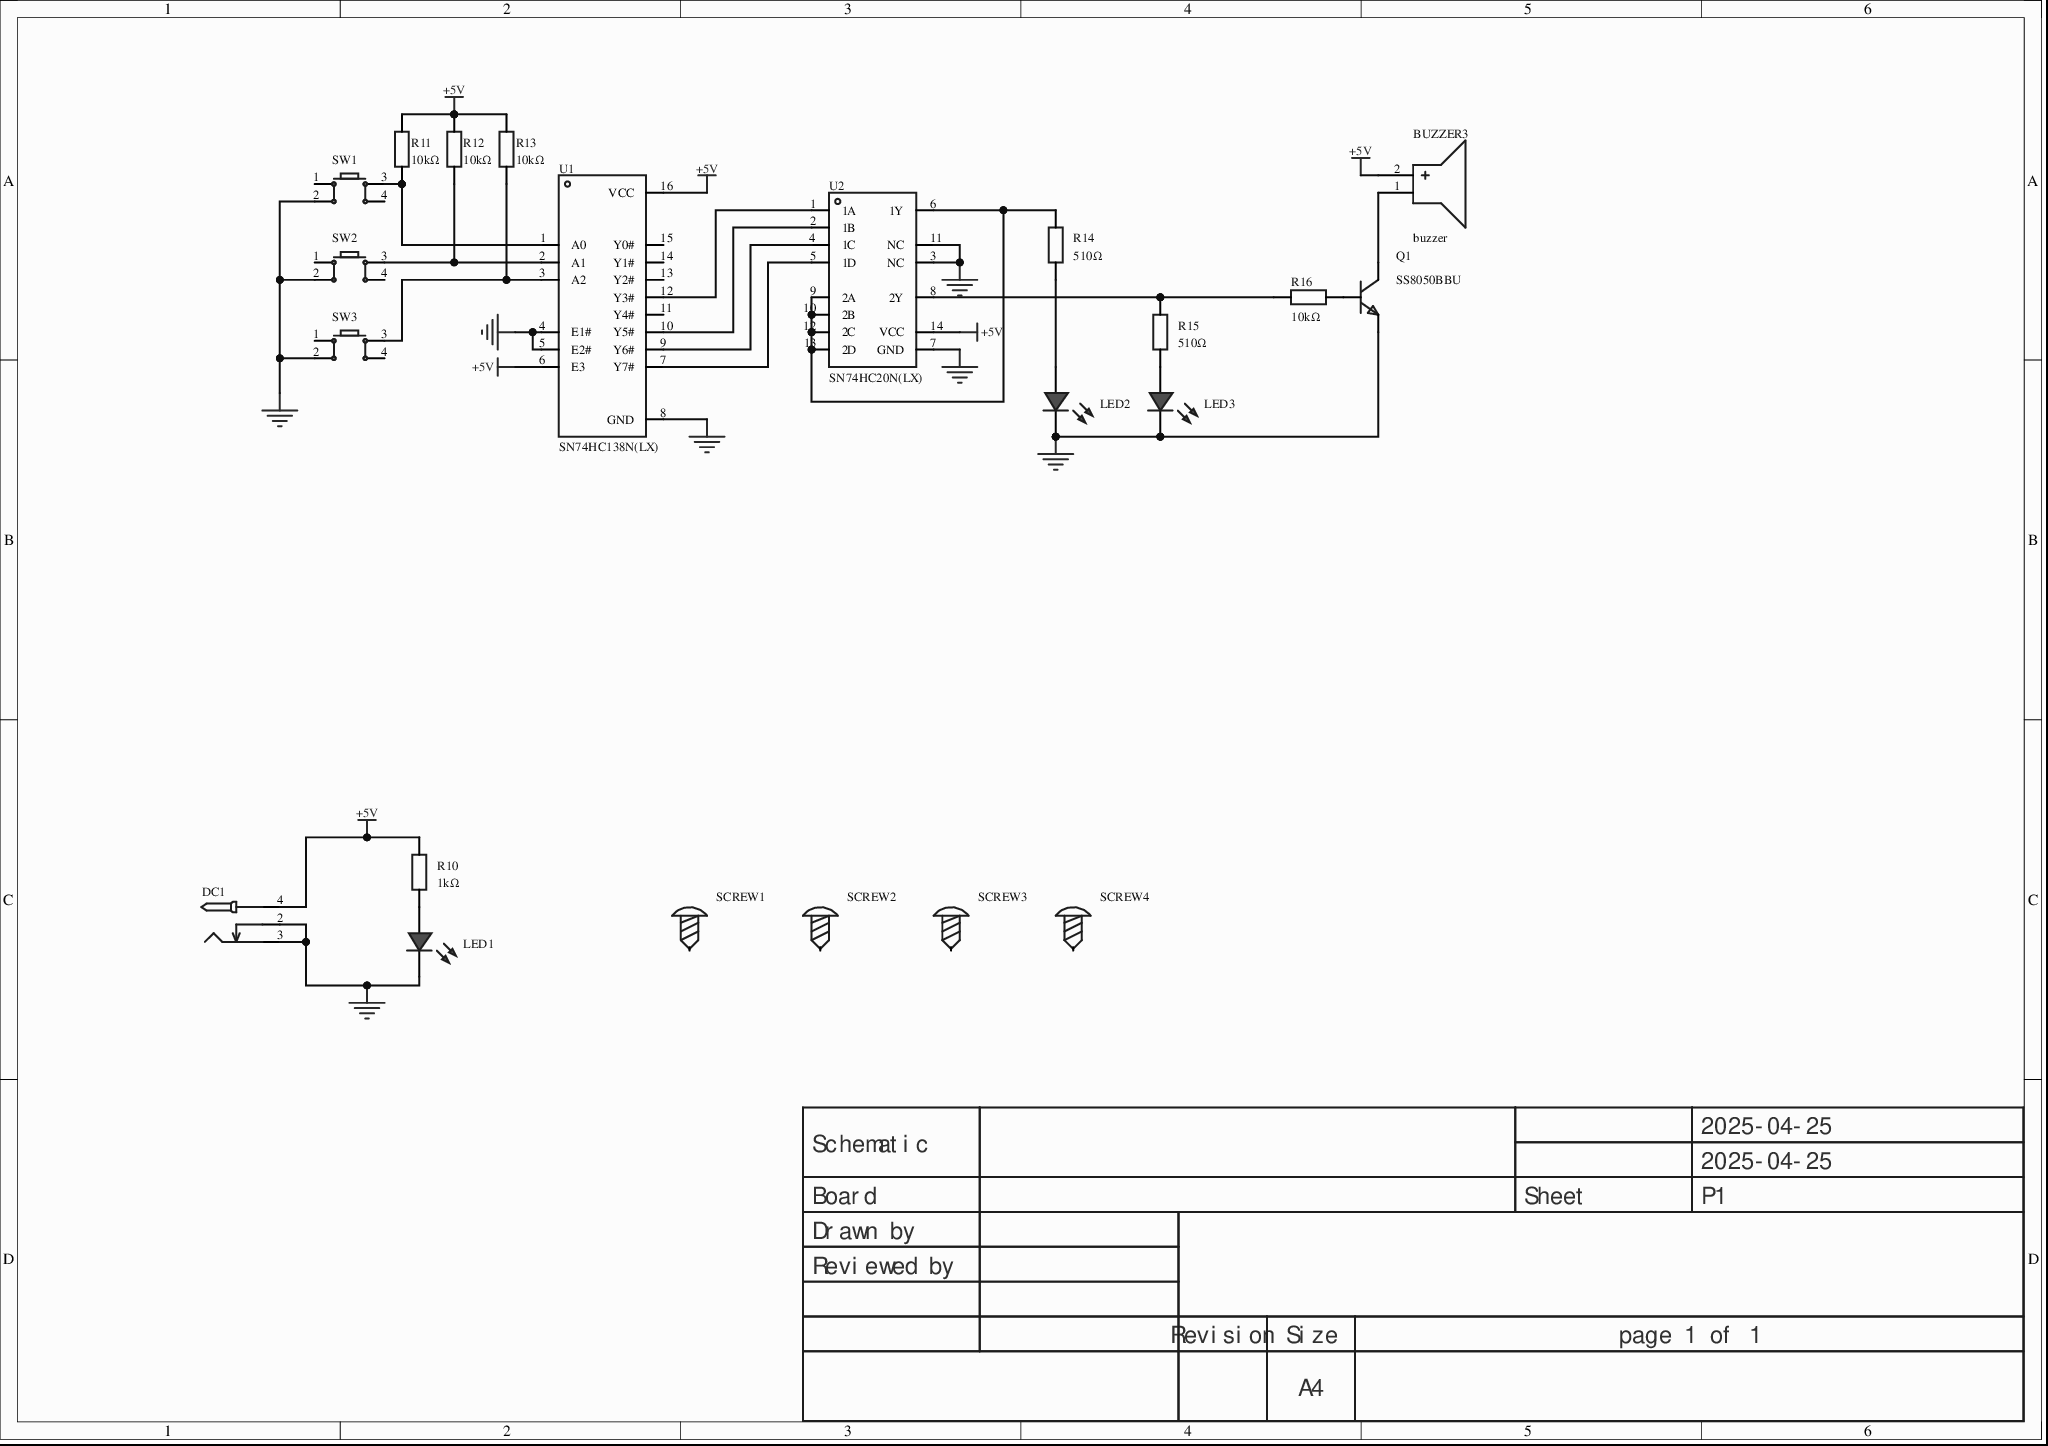
[diagram p0: MISC51615-3.schdoc]
# Altium project MISC51615-2.PrjPcb
1 sheet, 22 parts. Net scope: global (net labels, ports and power ports of the same name join across sheets).
Board file: MISC51615.pcbdoc

## Sheet MISC51615-3.schdoc
size 297 x 209 mm; Version: V1.0; @Project Name: MISC51615; @Page Count: 1; @Update Date: 2025-04-25; @Create Date: 2025-04-25; @Schematic Name: MISC51615; @Page No: 1; @Create Time: 10:35:49; @Update Time: 10:35:54; @Board Name: MISC51615

### Parts
BUZZER3  buzzer  [BUZ-TH_BD12.0-P6.00-D0.9-RD]
DC1  (no value)  [DC-2.0]
LED1  (no value)  [LED_TH-3mm]
LED2  (no value)  [LED_TH-3mm]
LED3  (no value)  [LED_TH-3mm]
Q1  SS8050BBU  [TO-92-3_L4.8-W3.7-P1.27-L-1]
R10  1kΩ  [Res_1/8W]
R11  10kΩ  [Res_1/8W]
R12  10kΩ  [Res_1/8W]
R13  10kΩ  [Res_1/8W]
R14  510Ω  [Res_1/8W]
R15  510Ω  [Res_1/8W]
R16  10kΩ  [Res_1/8W]
SCREW1  (no value)  [M3螺丝]
SCREW2  (no value)  [M3螺丝]
SCREW3  (no value)  [M3螺丝]
SCREW4  (no value)  [M3螺丝]
SW1  (no value)  [SW-TH_4P-L6.0-W6.0-P4.50-LS6.5]
SW2  (no value)  [SW-TH_4P-L6.0-W6.0-P4.50-LS6.5]
SW3  (no value)  [SW-TH_4P-L6.0-W6.0-P4.50-LS6.5]
U1  SN74HC138N(LX)  [PDIP-16_L19.3-W6.4-P2.54-LS7.94-BL]
U2  SN74HC20N(LX)  [PDIP-14_L19.3-W6.5-P2.54-LS7.6-BL]

### Nets
+5V: BUZZER3.2(+) DC1.4 R10.2 R11.2 R12.2 R13.2 U1.6(E3) U1.16(VCC) U2.14(VCC)
GND: DC1.2 DC1.3 LED1.2(A) LED2.2(A) LED3.2(A) Q1.1(E) SW1.2 SW2.2 SW3.2 U1.4(E1#) U1.5(E2#) U1.8(GND) U2.3(NC) U2.7(GND) U2.11(NC)
NetBUZZER3_1: BUZZER3.1(-) Q1.3(C)
NetLED1_1: LED1.1(C) R10.1
NetLED2_1: LED2.1(C) R14.1
NetLED3_1: LED3.1(C) R15.1
NetQ1_2: Q1.2(B) R16.2
NetR11_1: R11.1 SW1.3 U1.1(A0)
NetR12_1: R12.1 SW2.3 U1.2(A1)
NetR13_1: R13.1 SW3.3 U1.3(A2)
NetR14_2: R14.2 U2.6(1Y) U2.9(2A) U2.10(2B) U2.12(2C) U2.13(2D)
NetR15_2: R15.2 R16.1 U2.8(2Y)
NetU1_7: U1.7(Y7#) U2.5(1D)
NetU1_9: U1.9(Y6#) U2.4(1C)
NetU1_10: U1.10(Y5#) U2.2(1B)
NetU1_12: U1.12(Y3#) U2.1(1A)

Not connected (* = marked no-connect by the designer): SCREW1 1; SCREW2 1; SCREW3 1; SCREW4 1; SW1 1 4; SW2 1 4; SW3 1 4; U1 11(Y4#)* 13(Y2#)* 14(Y1#)* 15(Y0#)*

### Notes on the sheet
- 2025-04-25
- Schematic
- Board
- Sheet
- P1
- Drawn by
- Reviewed by
- Revision
- Size
- A4
- page 1 of 1

### Library data of the parts
BUZZER3 = buzzer: AddInBom: yes; ModelId: af17e4151ed84fc2a628230bf2376363; ModelTransform: 472.44,472.176,0,270,0,0,0,0,-196.85; Symbol: BUZZER; Device: buzzer; LCSC Part Name: buzzer; SupplierPart: C9900014030; ManufacturerPart: buzzer; Supplier Footprint: buzzer; JLCPCB Part Class: extended library; Supplier: LCSC; ConvertToPcb: yes; FootprintName: BUZ-TH_BD12.0-P6.00-D0.9-RD; ModelName: BUZ-TH_BD12.0-P6.00-D0.9-RD
DC1 = DC-005_2.0: ConvertToPcb: yes; SymbolName: DC power connector; ModelId: f5f20b8a2308479b936ba3c2698865bb0819f05c4eef4c71ace90d822a990e87; ModelName: DC-IN-TH_DC-5520-1; ModelTransform: 372.05,551.18,582.68,90,0,0,137.8,0,-149.61; Device: DC-005_2.0; AddInBom: yes; Supplier Footprint: 插件; FootprintName: DC-2.0
LED1-LED3 = LED_TH-R_3mm: ConvertToPcb: yes; ModelId: a497c992633541038a38947cdc58012f; ModelName: LED-TH-3mm_R; ModelTransform: 141.274,153.327,0,0,0,0,-5.984,0,-137.795; Symbol: LED_TH-R; Device: LED_TH-R_3mm; AddInBom: yes; FootprintName: LED_TH-3mm; Supplier Footprint: 插件
Q1 = SS8050BBU: Manufacturer: onsemi(安森美); AddInBom: yes; ModelId: 468dcd9de0d14f6892f8fd07a9314617; ModelTransform: 188.976,145.669,0,180,0,0,0,24.882,-196.85; Symbol: SS8050BBU; Device: SS8050BBU; LCSC Part Name: SS8050: NPN外延硅晶体管; SupplierPart: C5206368; ManufacturerPart: SS8050BBU; Supplier Footprint: TO-92-3; Datasheet: https://atta.szlcsc.com/upload/public/pdf/source/20221027/451CE33A66E14C75C6B6FE2D17BE4FB9.pdf; Supplier: LCSC; ConvertToPcb: yes; FootprintName: TO-92-3_L4.8-W3.7-P1.27-L-1; ModelName: TO-92-3_L4.8-W3.7-P1.27-L-1
R10-R16 = Res_AXIAL-1/8W: ConvertToPcb: yes; SymbolName: resistor; ModelId: b2b5ae7ae4c642178fe0039925c86a3f; ModelName: RES-TH_BD1.8-L3.2-P7.20-D0.4; ModelTransform: 282.86,66.88,253.09,0,0,0,0,0,-191; Device: Res_AXIAL-1/8W; AddInBom: yes; Supplier Footprint: 轴向引线; FootprintName: Res_1/8W
  R10: Value: 1kΩ
  R11-R13 R16: Value: 10kΩ
  R14 R15: Value: 510Ω
SCREW1-SCREW4 = M3螺丝: Device: M3 screw; ConvertToPcb: yes; SymbolName: screw hole; AddInBom: yes; Supplier Footprint: 插件; FootprintName: M3 screw
SW1-SW3 = Key_TH_6x6x6: Contact current:50mA; rated voltage (DC):12V; insulation resistance:100MΩ; circuit structure: SPST; mounting: through-hole; button shape: round button; button/cap colour: black; operating force: 260gf@±30gf; operating temperature: -25℃~+70℃; pin style: PC pin; switch length: 6mm; switch width: 6mm; switch height: 6mm; with bracket: no;; Symbol: tactile switch; ConvertToPcb: yes; ModelId: 20eee248bc684ccd8cbdbb1d0d91ec6f; ModelName: SW-TH_4P-L6.0-W6.0-H5.0-LS6.5-P4.50; ModelTransform: 236.22,323.03,0,90,0,0,0,0,-137.795; Device: Key_TH_6x6x6; AddInBom: yes; SupplierPart: C2837516; Supplier Footprint: 插件; FootprintName: SW-TH_4P-L6.0-W6.0-P4.50-LS6.5
U1 = SN74HC138N(LX): Operating voltage: 2V~6V;; Manufacturer: LX(灵星芯微); AddInBom: yes; ModelId: 96ff5d01b3074dd183bcbc4cd00a63de; ModelTransform: 759.841,322.44,0,0,0,0,0,0,-137.795; Voltage Supply Source: single supply; Symbol: SN74HC138N(LX); Device: SN74HC138N(LX); LCSC Part Name: 集成电路; SupplierPart: C22436652; ManufacturerPart: SN74HC138N(LX); Supplier Footprint: DIP-16; JLCPCB Part Class: extended library; Datasheet: https://atta.szlcsc.com/upload/public/pdf/source/20240524/CB21E824929BADE59169C0B1043B57DD.pdf; Supplier: LCSC; ConvertToPcb: yes; FootprintName: PDIP-16_L19.3-W6.4-P2.54-LS7.94-BL; ModelName: PDIP-16_L19.3-W6.4-P2.54-LS7.94-BL; Type: decoder/demultiplexer; Voltage - Supply: 2V~6V; Operating temperature: -
U2 = SN74HC20N(LX): Logic type: NAND gate; channels: 2; operating voltage: 2V~6V; quiescent current (Iq): 2uA; propagation delay (tpd): 15ns@6V,50pF;; Manufacturer: LX(灵星芯微); AddInBom: yes; ModelId: 7604059b31ae49f98a0332a7cce2343e; ModelTransform: 759.15391,311.417,0,0,0,0,0,0,-129.921; Number of Channels: 2; Input Logic Level - High: 1.5V~4.2V; Input Logic Level - Low: 500mV~1.8V; Symbol: SN74HC20N(LX); Device: SN74HC20N(LX); LCSC Part Name: SN74HC20N(LX); SupplierPart: C22449652; ManufacturerPart: SN74HC20N(LX); Supplier Footprint: DIP-14; Datasheet: https://atta.szlcsc.com/upload/public/pdf/source/20240603/8583561A4517AE1122D991330CF9FCE0.pdf; Supplier: LCSC; ConvertToPcb: yes; FootprintName: PDIP-14_L19.3-W6.5-P2.54-LS7.6-BL; ModelName: PDIP-14_L19.3-W6.5-P2.54-LS7.6-BL; Logic Type: NAND gate; Voltage - Supply: 2V~6V; Quiescent Current: 2uA; Series: 74HC series; Propagation Delay: 15ns@6V,50pF; Operating Temperature: -40℃~+105℃